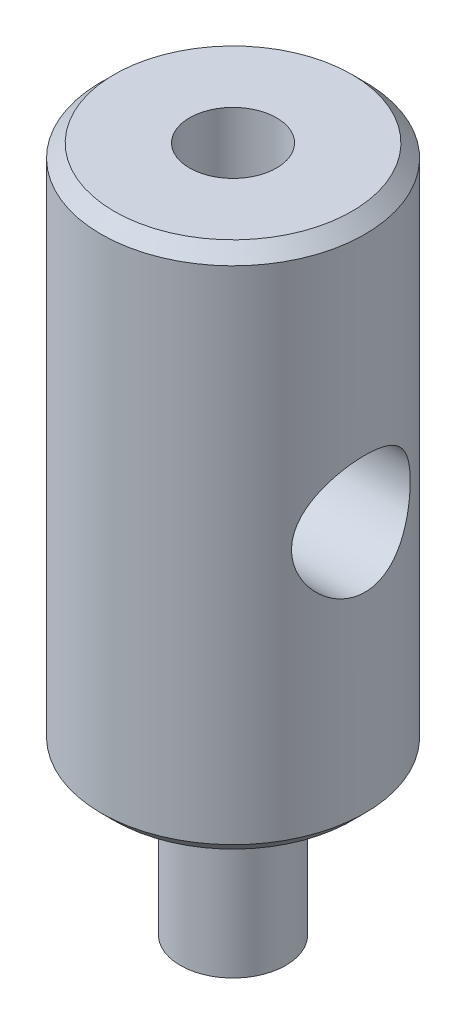
SolidWorks part; units mm, degrees
ref_plane "前视" through (0, 0, 0) normal (0, 0, 1) x (1, 0, 0)
ref_plane "上视" through (0, 0, 0) normal (0, 1, 0) x (1, 0, 0)
ref_plane "右视" through (0, 0, 0) normal (1, 0, 0) x (0, 0, -1)
sketch "草图1" plane through (0, 0, 0) normal (0, 1, 0) x (1, 0, 0)
  circle A0 centre (0, 0) radius 5
  dimension "D1" = 10
extrude "凸台-拉伸1" add sketch "草图1" along normal mid plane 20
sketch "草图2" plane through (0, -10, 0) normal (0, -1, 0) x (1, 0, 0)
  circle A0 centre (0, 0) radius 2
  dimension "D1" = 4
extrude "凸台-拉伸2" add sketch "草图2" along normal blind 6
cosmetic thread "装饰螺纹线1" parameters "D1"=5.5, "D2"=3.3
sketch "草图3" plane through (0, 0, 0) normal (0, 0, 1) x (1, 0, 0)
  line L0 (2, -16) -> (2, -10) construction
  line L1 (1.7, -10) -> (2, -10)
  line L2 (1.7, -10) -> (1.7, -10.5)
  line L3 (1.7, -10.5) -> (2, -10.5)
  line L4 (2, -10) -> (2, -10.5)
  line L5 (-2, -10) -> (2, -10) construction
  line L6 (0, 0) -> (0, -26.8399) construction
  dimension "D1" = 0.5
  dimension "D2" = 0.3
revolve "切除-旋转1" cut sketch "草图3" angle 360 about L6
hole_wizard "M4 螺纹孔1" positions "草图5" profile "草图4" tap size "M4" standard "Gb"
sketch "草图5" plane through (0, 10, 0) normal (0, 1, 0) x (1, 0, 0)
  point P0 (0, 0)
sketch "草图4" plane through (0, 10, 0) normal (1, 0, 0) x (0, 0, 1)
  line L0 (0, 0) -> (0, 11.0914)
  line L1 (0, 11.0914) -> (1.65, 10.1)
  line L2 (1.65, 10.1) -> (1.65, 0)
  line L5 (1.65, 0) -> (0, 0)
  line L10 (0, 11.0914) -> (-1.65, 10.1) construction
  line L11 (0, -6.35) -> (0, 107.95) construction
  dimension "螺纹孔钻头直径" = 3.3
  dimension "螺纹孔钻头深度" = 10.1
  dimension "导头角度" = 118
cosmetic thread "孔螺蚊线1" parameters "D1"=8, "D2"=4
chamfer "倒角1" distance 0.5 angle 45 2 edges at (0, 10, 5) (0, -10, 5)
sketch "草图6" plane through (0, 0, 0) normal (1, 0, 0) x (0, 0, -1)
  circle A0 centre (0, 0) radius 2.25
  dimension "D1" = 4.5
extrude "切除-拉伸1" cut sketch "草图6" against normal through all and the other way through all
